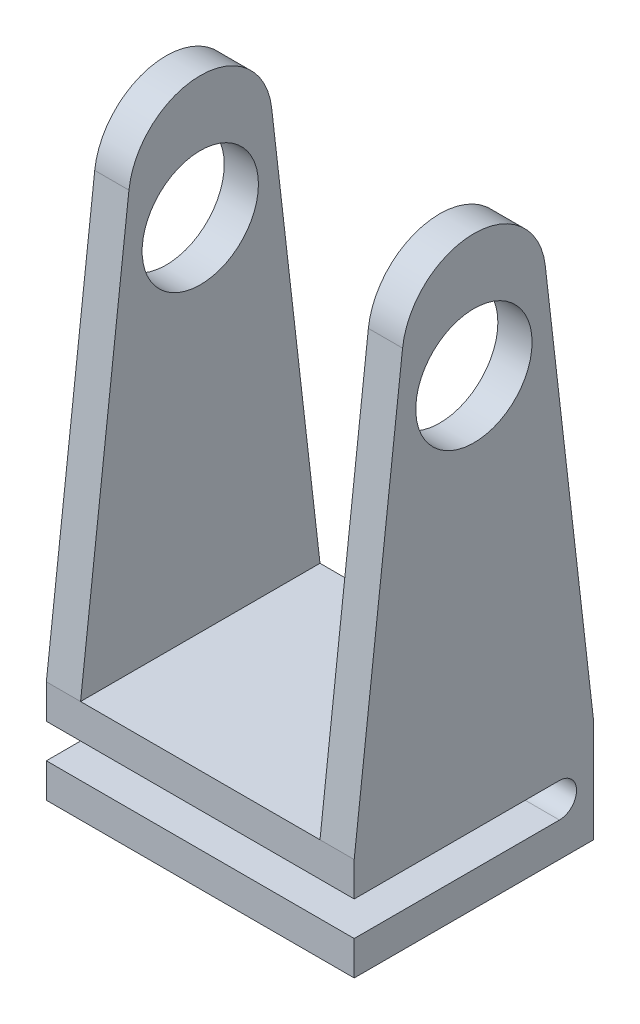
from build123d import *

# Parameters (mm, degrees)
SKETCH1_W           = 90
SKETCH1_H           = 70
BOSS_EXTRUDE1_DEPTH = 30
SKETCH2_R           = 17
BOSS_EXTRUDE2_DEPTH = 10
CUT_EXTRUDE1_DEPTH  = 197.38228026


with BuildPart() as part:
    # Sketch1 → Boss-Extrude1 (new body)
    with BuildSketch(Plane(origin=(0, 0, 0), x_dir=(1, 0, 0), z_dir=(0, 1, 0))):
        Rectangle(SKETCH1_W, SKETCH1_H)
    extrude(amount=BOSS_EXTRUDE1_DEPTH)

    # Sketch2 → Boss-Extrude2 (add)
    with BuildSketch(Plane(origin=(45, 0, 0), x_dir=(0, 0, -1), z_dir=(1, 0, 0))):
        with BuildLine():
            Line((-20.861305824, 152.409547532), (-35, 30))
            Line((-35, 30), (35, 30))
            Line((35, 30), (20.861305824, 152.409547532))
            ThreePointArc((20.861305824, 152.409547532), (0, 171), (-20.861305824, 152.409547532))
        make_face()
        with Locations((0, 135)):
            Circle(SKETCH2_R, mode=Mode.SUBTRACT)
    boss_extrude2 = extrude(amount=-BOSS_EXTRUDE2_DEPTH)

    # Mirror1: Boss-Extrude2 across plane
    add(boss_extrude2.mirror(Plane(origin=(0, 0, 0), x_dir=(0, 0, 1), z_dir=(1, 0, 0))))

    # Sketch3 → Cut-Extrude1 (cut, through all)
    with BuildSketch(Plane(origin=(45, 0, 0), x_dir=(0, 0, -1), z_dir=(1, 0, 0))):
        with BuildLine():
            Line((25, 20), (-35, 20))
            Line((-35, 20), (-35, 10))
            Line((-35, 10), (25, 10))
            ThreePointArc((25, 10), (20, 15), (25, 20))
        make_face()
        with BuildLine():
            ThreePointArc((30, 15), (28.535533906, 18.535533906), (25, 20))
            Line((25, 20), (25, 10))
            ThreePointArc((25, 10), (28.535533906, 11.464466094), (30, 15))
        make_face()
        with BuildLine():
            Line((25, 10), (25, 20))
            ThreePointArc((25, 20), (20, 15), (25, 10))
        make_face()
    extrude(amount=-CUT_EXTRUDE1_DEPTH, mode=Mode.SUBTRACT)


solid = part.part
